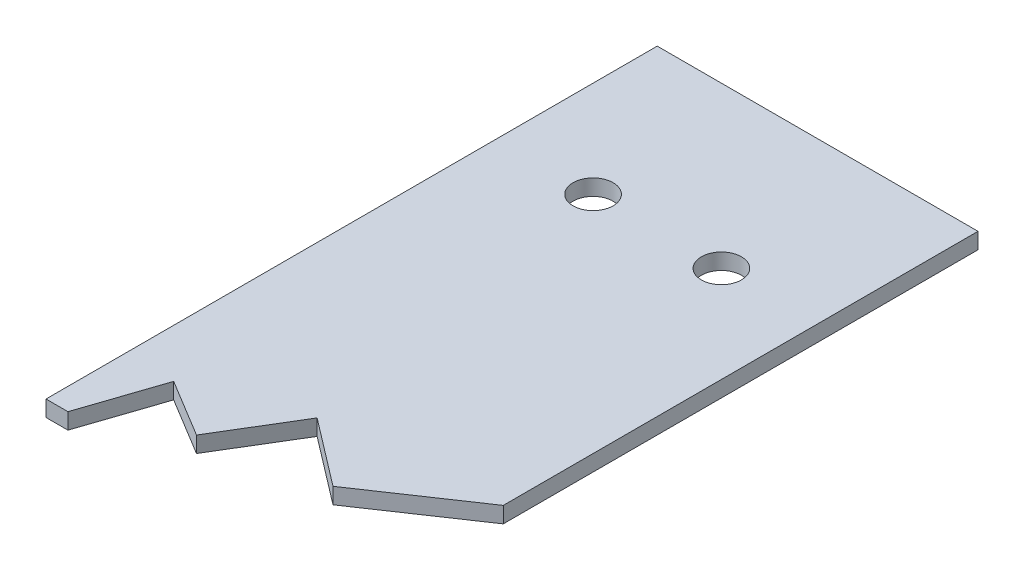
from build123d import *

# Parameters (mm, degrees)
SKETCH1_W           = 40
SKETCH1_H           = 80
BOSS_EXTRUDE1_DEPTH = 2
SKETCH2_R           = 2.5
CUT_EXTRUDE1_DEPTH  = 10
CUT_EXTRUDE2_DEPTH  = 10


with BuildPart() as part:
    # Sketch1 → Boss-Extrude1 (new body)
    with BuildSketch(Plane(origin=(0, 0, 0), x_dir=(1, 0, 0), z_dir=(0, 1, 0))):
        Rectangle(SKETCH1_W, SKETCH1_H)
    extrude(amount=BOSS_EXTRUDE1_DEPTH)

    # Sketch2 → Cut-Extrude1 (cut)
    with BuildSketch(Plane.XZ):
        with Locations(Location((8, -20, 0), (0, 0, 270))):
            Circle(SKETCH2_R)
        with Locations(Location((-8, -20, 0), (0, 0, 270))):
            Circle(SKETCH2_R)
    extrude(amount=-CUT_EXTRUDE1_DEPTH, mode=Mode.SUBTRACT)

    # Sketch3 → Cut-Extrude2 (cut)
    with BuildSketch(Plane(origin=(0, 2, 0), x_dir=(1, 0, 0), z_dir=(0, 1, 0))):
        Polygon((20, -19.19837027), (7.322915473, -27.754938711), (-1.053514684, -21.360029666), (-6.727870598, -30.72722038), (-13.940955905, -26.357755241), (-17.265960151, -36.22143801), (-20, -36.22143801), (-20, -40), (20, -40), align=None)
    extrude(amount=-CUT_EXTRUDE2_DEPTH, mode=Mode.SUBTRACT)


solid = part.part
